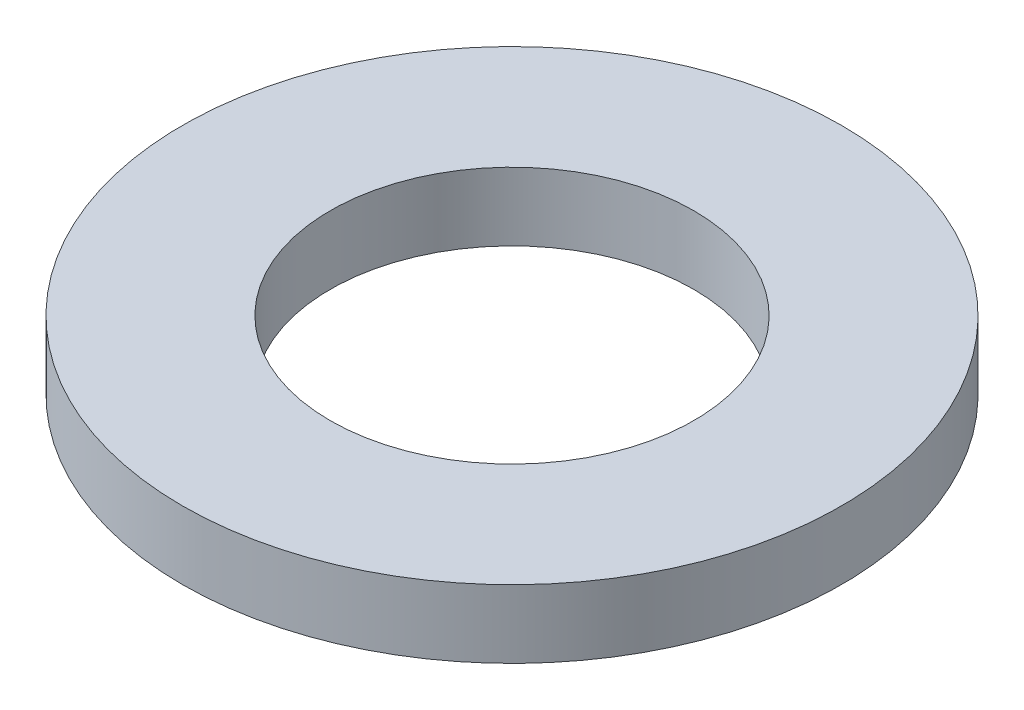
from build123d import *

# Parameters (mm, degrees)
SKETCH_1_R      = 5.8
SKETCH_1_R_2    = 3.2
EXTRUDE_1_DEPTH = 1.2


with BuildPart() as part:
    # 草图1 → 凸台-拉伸1 (new body)
    with BuildSketch(Plane(origin=(0, 0, 0), x_dir=(1, 0, 0), z_dir=(0, 1, 0))):
        with Locations(Location((0, 0, 0), (0, 0, 270))):
            Circle(SKETCH_1_R)
        with Locations(Location((0, 0, 0), (0, 0, 270))):
            Circle(SKETCH_1_R_2, mode=Mode.SUBTRACT)
    extrude(amount=EXTRUDE_1_DEPTH)


solid = part.part
